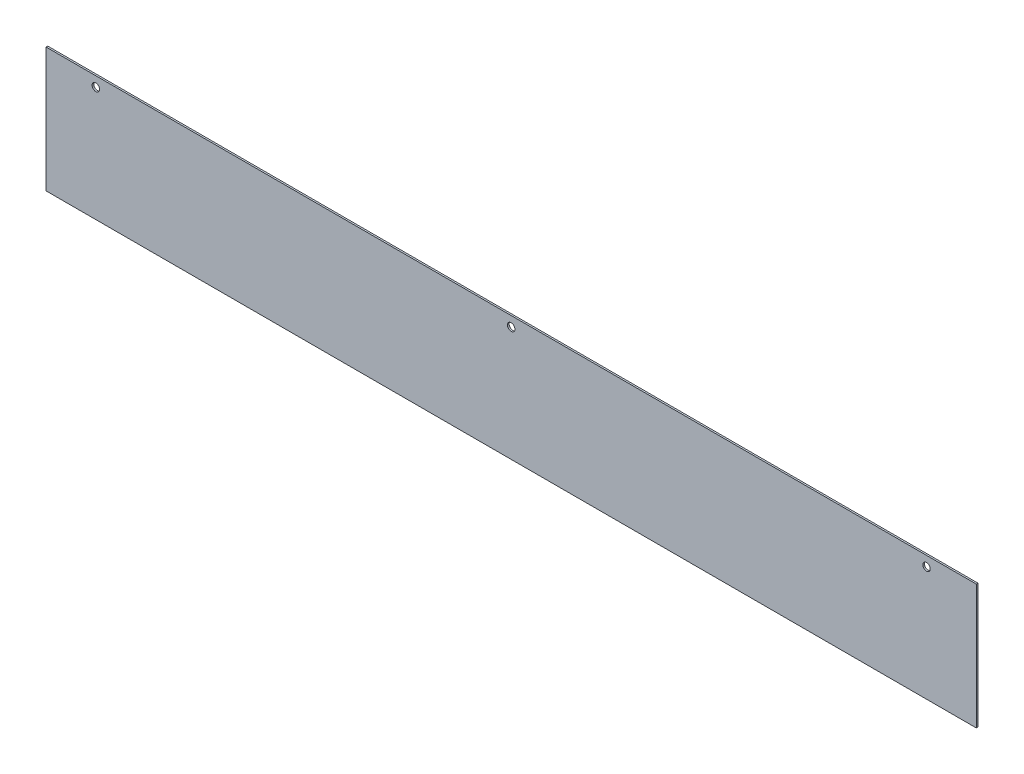
from build123d import *

# Parameters (mm, degrees)
SKETCH1_W          = 560
SKETCH1_H          = 1
EXTRUDE1_DEPTH     = 37.5
SKETCH3_R          = 2.25
CUT_EXTRUDE1_DEPTH = 283.501769906


with BuildPart() as part:
    # Sketch1 → Extrude1 (new, symmetric)
    with BuildSketch(Plane(origin=(0, 0, 0), x_dir=(1, 0, 0), z_dir=(0, 1, 0))):
        Rectangle(SKETCH1_W, SKETCH1_H)
    extrude(amount=EXTRUDE1_DEPTH, both=True)

    # Sketch3 → Cut-Extrude1 (cut, through all)
    with BuildSketch(Plane.XY.offset(0.5)):
        with Locations((-250, 31.5)):
            Circle(SKETCH3_R)
        with Locations(Location((250, 31.5, 0), (0, 0, 180))):
            Circle(SKETCH3_R)
        with Locations((0, 31.5)):
            Circle(SKETCH3_R)
    extrude(amount=-CUT_EXTRUDE1_DEPTH, mode=Mode.SUBTRACT)


solid = part.part
